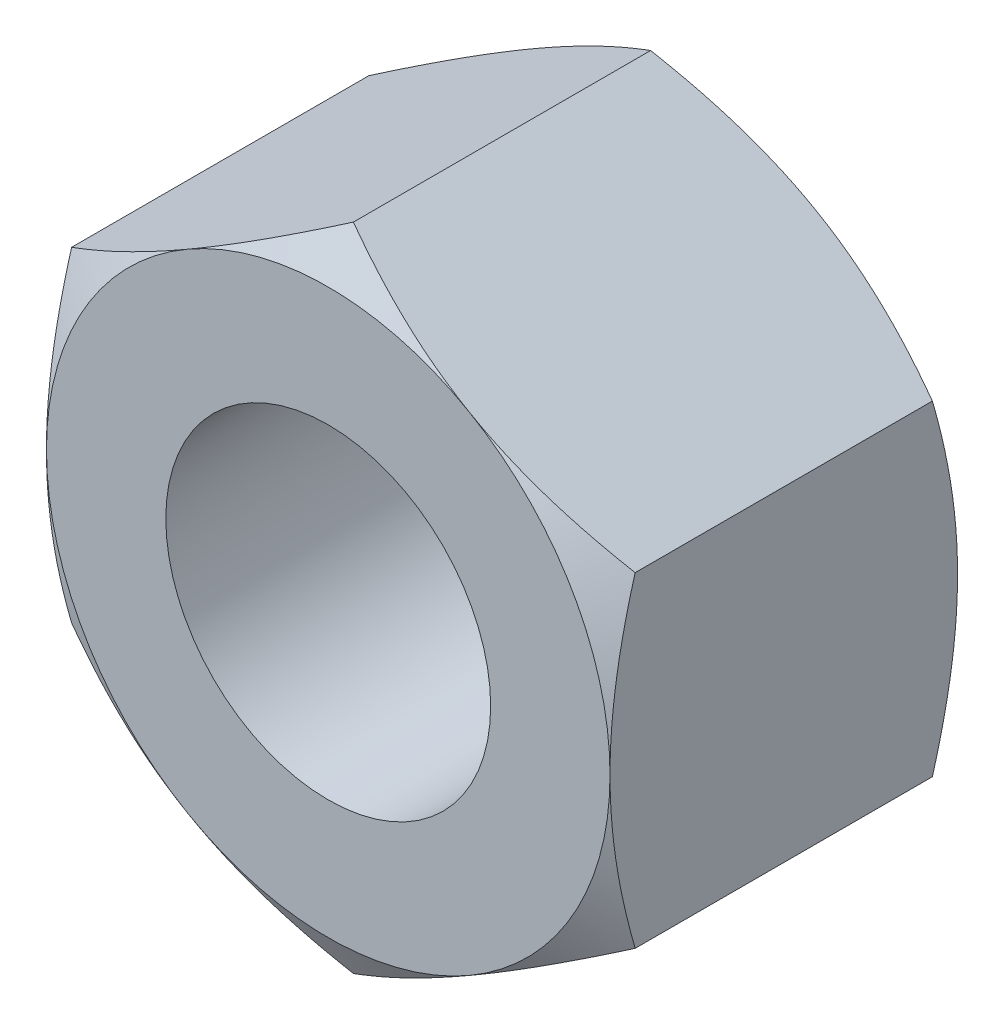
SolidWorks part; units mm, degrees
ref_plane "基准面1" through (0, 0, 0) normal (0, 0, 1) x (1, 0, 0)
ref_plane "基准面2" through (0, 0, 0) normal (0, 1, 0) x (1, 0, 0)
ref_plane "基准面3" through (0, 0, 0) normal (1, 0, 0) x (0, 0, -1)
sketch "尺寸草图" plane through (0, 0, 0) normal (0, 0, 1) x (1, 0, 0)
  line L0 (0, 0) -> (26.8, 0) construction
  line L1 (0, 0) -> (53.6, 0) construction
  line L2 (26.8, 0) -> (49.3, 0) construction
  line L3 (-15.2381, 0) -> (0, 0) construction
  point P3 (16, 0)
  point P4 (2, 0)
  point P5 (26.8, 0)
  point P6 (14.8, 0)
  point P8 (24, 0)
  dimension "D1" = 15.2381
  dimension "D" = 16
  dimension "P" = 2
  dimension "e(最小)" = 26.8
  dimension "m(最大)" = 14.8
  dimension "s(公称)" = 24
  dimension "dw(最小)" = 22.5
sketch "草图1" plane through (0, 0, 0) normal (0, 0, 1) x (1, 0, 0)
  line L0 (-12, 0) -> (12, 0) construction
  line L1 (0, 13.8564) -> (0, -13.8564) construction
  line L3 (0, 13.8564) -> (-12, 6.9282)
  line L4 (-12, 6.9282) -> (-12, -6.9282)
  line L5 (-12, -6.9282) -> (0, -13.8564)
  line L6 (0, -13.8564) -> (12, -6.9282)
  line L7 (12, -6.9282) -> (12, 6.9282)
  line L8 (12, 6.9282) -> (0, 13.8564)
  circle A0 centre (0, 0) radius 12 construction
  circle A1 centre (0, 0) radius 6.9175
  point P2 (0, 12.9436)
  dimension "D1" = 26.8
  dimension "D" = 13.835
  dimension "D2" = 24
extrude "基体-拉伸" add sketch "草图1" along normal blind 14.8
cosmetic thread "装饰螺纹线1" parameters "D2"=16
sketch "草图2" plane through (0, 0, 0) normal (0, 0, -1) x (-1, 0, 0)
  circle A0 centre (0, 0) radius 12
  circle A1 centre (0, 0) radius 6.9175 construction
  dimension "s" = 24
extrude "切除-拉伸1" cut sketch "草图2" against normal through all draft 60 flip side to cut
sketch "草图3" plane through (0, 0, 14.8) normal (0, 0, 1) x (1, 0, 0)
  circle A0 centre (0, 0) radius 12
  dimension "D1" = 24
extrude "切除-拉伸2" cut sketch "草图3" against normal through all draft 60 flip side to cut
